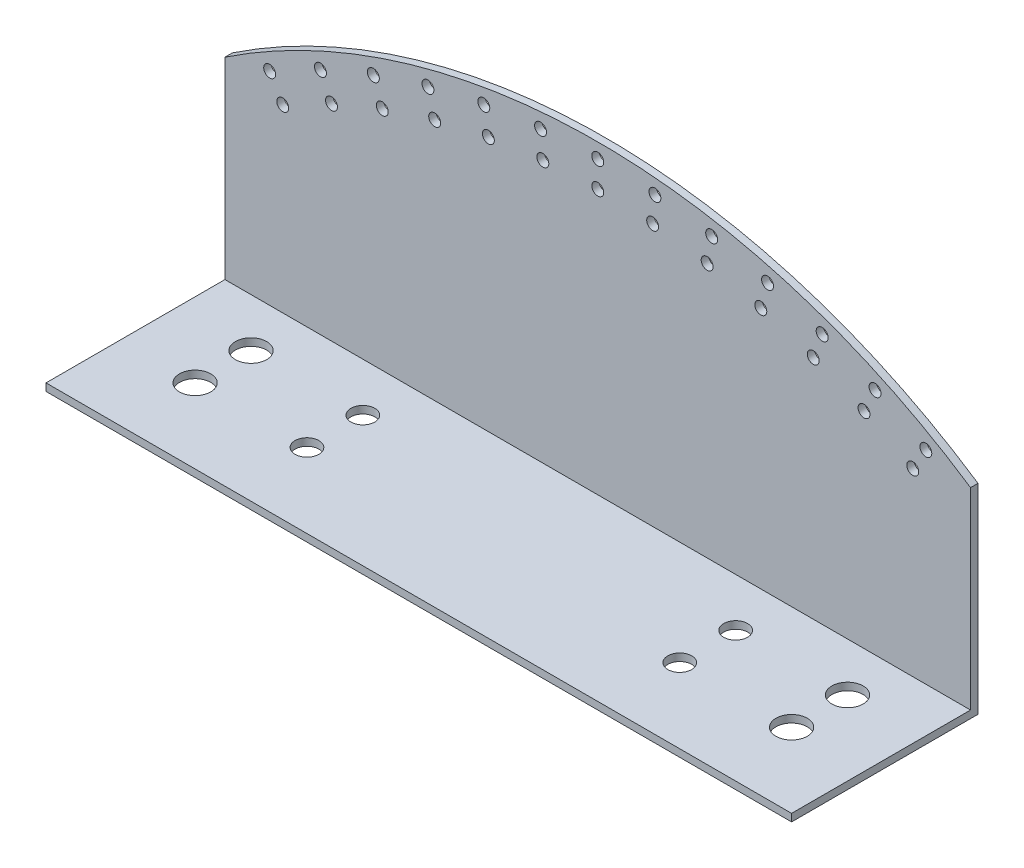
SolidWorks part; units mm, degrees
ref_plane "前视基准面" through (0, 0, 0) normal (0, 0, 1) x (1, 0, 0)
ref_plane "上视基准面" through (0, 0, 0) normal (0, 1, 0) x (1, 0, 0)
ref_plane "右视基准面" through (0, 0, 0) normal (1, 0, 0) x (0, 0, -1)
sketch "草图1" plane through (0, 0, 0) normal (0, 0, 1) x (1, 0, 0)
  line L0 (1437.2737, 307.4801) -> (1237.2737, 307.4801)
  line L2 (1437.2737, 307.4801) -> (1437.2737, 361.1464)
  line L3 (1237.2737, 307.4801) -> (1237.2737, 361.1464)
  arc A0 (1437.2737, 361.1464) -> (1237.2737, 361.1464) centre (1337.2737, 211.4801) ccw
  arc A1 (1437.2737, 356.311) -> (1237.2737, 356.311) centre (1337.2737, 211.4801) ccw construction
  arc A2 (1437.2737, 347.7189) -> (1237.2737, 347.7189) centre (1337.2737, 211.4801) ccw construction
  circle A3 centre (1337.2737, 387.4801) radius 1.6
  circle A4 centre (1337.2737, 380.4801) radius 1.6
  circle A5 centre (1321.9343, 386.8104) radius 1.6
  circle A6 centre (1322.5444, 379.837) radius 1.6
  circle A7 centre (1306.7116, 384.8063) radius 1.6
  circle A8 centre (1307.9272, 377.9126) radius 1.6
  circle A9 centre (1291.7216, 381.4831) radius 1.6
  circle A10 centre (1293.5333, 374.7216) radius 1.6
  circle A11 centre (1277.0782, 376.866) radius 1.6
  circle A12 centre (1279.4723, 370.2882) radius 1.6
  circle A13 centre (1262.8929, 370.9903) radius 1.6
  circle A14 centre (1265.8512, 364.6461) radius 1.6
  circle A15 centre (1249.2737, 363.9006) radius 1.6
  circle A16 centre (1252.7737, 357.8384) radius 1.6
  circle A17 centre (1425.2737, 363.9006) radius 1.6
  circle A18 centre (1421.7737, 357.8384) radius 1.6
  circle A19 centre (1411.6545, 370.9903) radius 1.6
  circle A20 centre (1408.6962, 364.6461) radius 1.6
  circle A21 centre (1397.4693, 376.866) radius 1.6
  circle A22 centre (1395.0751, 370.2882) radius 1.6
  circle A23 centre (1382.8259, 381.4831) radius 1.6
  circle A24 centre (1381.0141, 374.7216) radius 1.6
  circle A25 centre (1367.8358, 384.8063) radius 1.6
  circle A26 centre (1366.6203, 377.9126) radius 1.6
  circle A27 centre (1352.6131, 386.8104) radius 1.6
  circle A28 centre (1352.003, 379.837) radius 1.6
extrude "凸台-拉伸1" add sketch "草图1" along normal blind 2
sketch "草图2" plane through (0, 0, 2) normal (0, 0, 1) x (1, 0, 0)
  line L0 (1437.2737, 307.4801) -> (1437.2737, 361.1464) construction
  line L1 (1237.2737, 307.4801) -> (1437.2737, 307.4801)
  line L2 (1237.2737, 307.4801) -> (1237.2737, 309.4801)
  line L3 (1237.2737, 309.4801) -> (1437.2737, 309.4801)
  line L4 (1437.2737, 307.4801) -> (1437.2737, 309.4801)
  dimension "D1" = 2
extrude "凸台-拉伸2" add sketch "草图2" along normal blind 48
sketch "草图3" plane through (0, 309.4801, 0) normal (0, 1, 0) x (1, 0, 0)
  line L0 (1437.2737, -50) -> (1237.2737, -50) construction
  line L1 (1437.2737, -30) -> (1237.2737, -30) construction
  line L2 (1437.2737, -15) -> (1237.2737, -15) construction
  circle A0 centre (1287.2737, -30) radius 3.2
  circle A1 centre (1387.2737, -30) radius 3.2
  circle A2 centre (1257.2737, -15) radius 4.2
  circle A3 centre (1417.2737, -15) radius 4.2
  circle A4 centre (1257.2737, -30) radius 4.2
  circle A5 centre (1287.2737, -15) radius 3.2
  circle A6 centre (1387.2737, -15) radius 3.2
  circle A7 centre (1417.2737, -30) radius 4.2
extrude "切除-拉伸1" cut sketch "草图3" against normal blind 48
